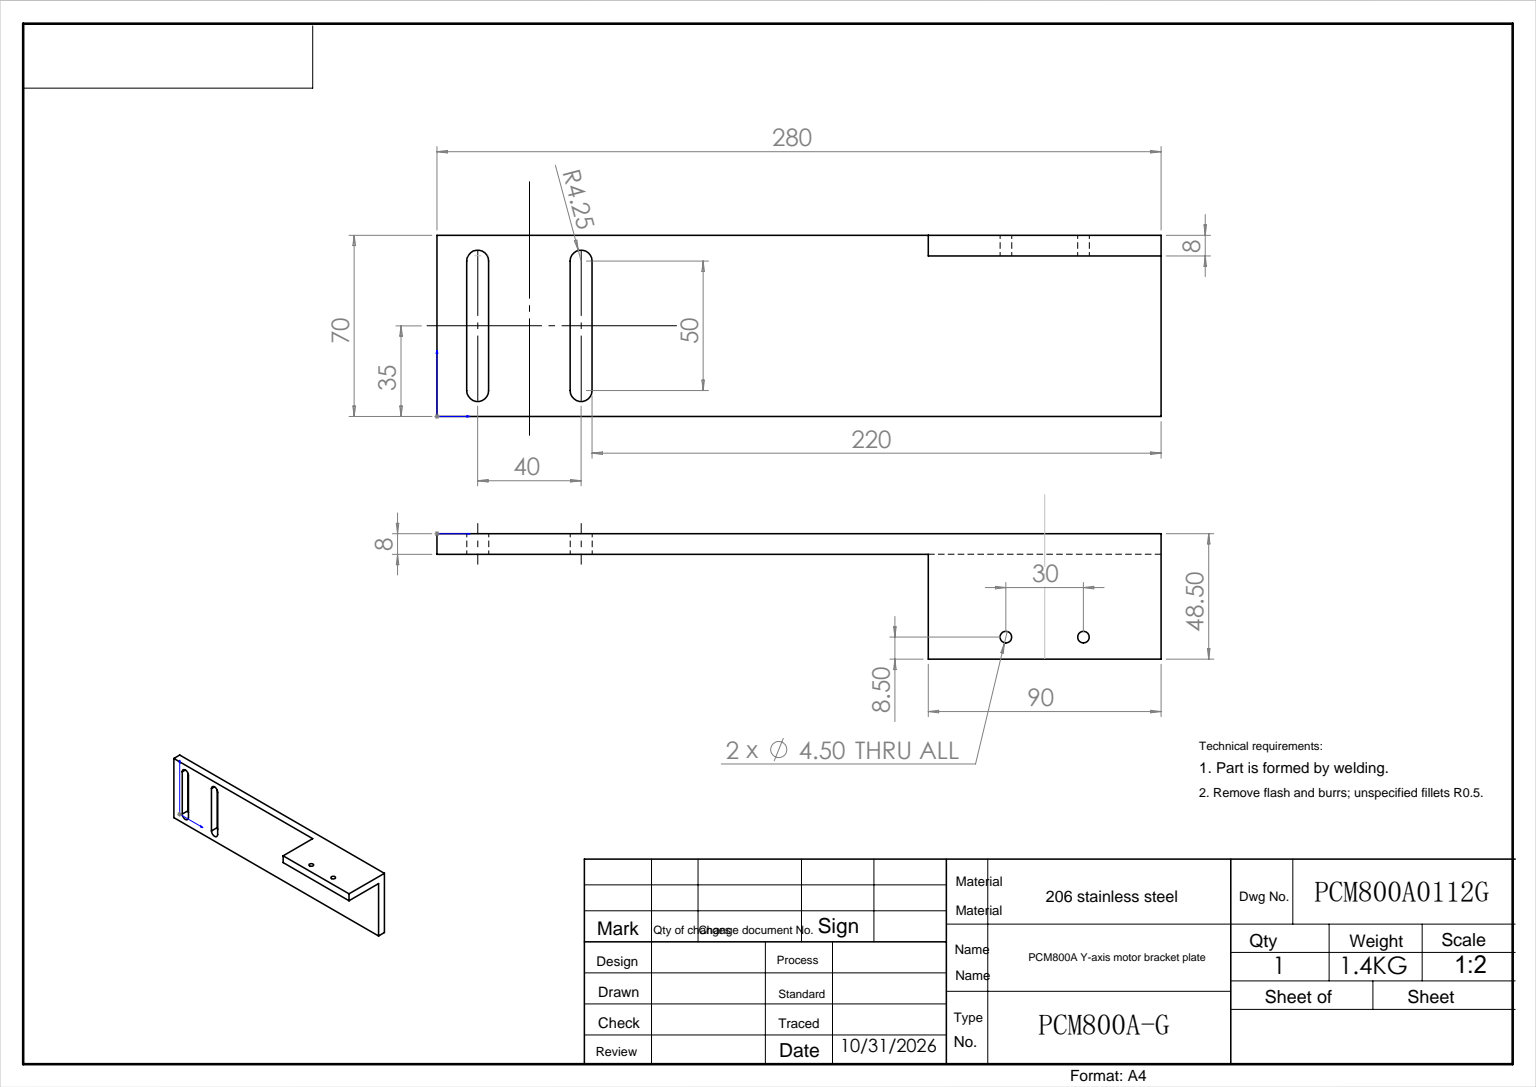
from build123d import *

# Parameters (mm, degrees)
SKETCH_1_W              = 280
SKETCH_1_H              = 70
EXTRUDE_1_DEPTH         = 8
SKETCH_2_W              = 90
SKETCH_2_H              = 8
EXTRUDE_2_DEPTH         = 40.5
HOLE_WIZARD_4_5_4_5_1_D = 4.5


with BuildPart() as part:
    # 草图1 → 凸台-拉伸1 (new body)
    with BuildSketch(Plane.XY):
        with Locations((140, 35)):
            Rectangle(SKETCH_1_W, SKETCH_1_H)
        with BuildLine():
            Line((51.5, 60), (51.5, 10))
            ThreePointArc((51.5, 10), (55.75, 5.75), (60, 10))
            Line((60, 10), (60, 60))
            ThreePointArc((60, 60), (55.75, 64.25), (51.5, 60))
        make_face(mode=Mode.SUBTRACT)
        with BuildLine():
            Line((11.5, 60), (11.5, 10))
            ThreePointArc((11.5, 10), (15.75, 5.75), (20, 10))
            Line((20, 10), (20, 60))
            ThreePointArc((20, 60), (15.75, 64.25), (11.5, 60))
        make_face(mode=Mode.SUBTRACT)
    extrude(amount=EXTRUDE_1_DEPTH)

    # 草图2 → 凸台-拉伸2 (add)
    with BuildSketch(Plane.XY.offset(8)):
        with Locations((235, 66)):
            Rectangle(SKETCH_2_W, SKETCH_2_H)
    extrude(amount=EXTRUDE_2_DEPTH)

    # Ø4.5 (4.5) 直径孔1 (through all)
    with Locations(Plane(origin=(0, 70, 0), x_dir=(-1, 0, 0), z_dir=(0, 1, 0))):
        with Locations((-220, 40), (-250, 40)):
            Hole(HOLE_WIZARD_4_5_4_5_1_D / 2)


solid = part.part
